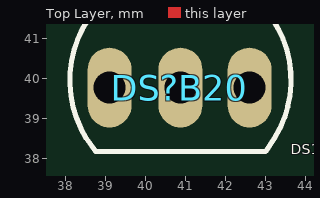
[diagram p0: Top Layer view]
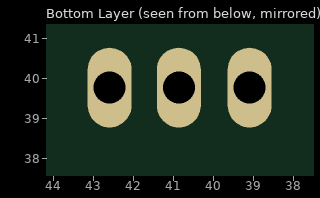
[diagram p1: Bottom Layer view, seen from below]
# Altium PCB MISC84237-4.PcbDoc
Units mm, origin at the board's own origin, x right, y up, seen from the top; angles counter-clockwise.
Board outline 32.45 x 30.27 mm, 2 copper layers (Top Layer, Bottom Layer); 1 components, 0 nets, 3 pads, 0 vias.

## Layer stack, top to bottom (the 12.6 mil dielectric is the usual default, probably not edited)
Top Layer: signal copper (thickness not stored)
Dielectric: dielectric 0.32, FR-4, Dk 4.8
Bottom Layer: signal copper (thickness not stored)

## Board outline
57.852,25.4 25.4,25.4 25.4,55.668 57.852,55.668

## Components (designator, comment, footprint, x,y, rotation, side; value= is the part's Value field where it differs from the comment)
DS?B20 "DS18B20 temperature sensor" DS18B20温度传感器 40.864,40.407 r0 top

## Footprints (in the part's own frame and the unit in brackets; to place one, negate y for a bottom-side part, rotate by r counter-clockwise, add the part's x,y. Pads: shape width x height; smd on the part's side, far side on the other; paste and mask are expansions set on the pad)
DS18B20温度传感器 [mm]
  oval 1.1x2 hole 0.8 paste+0 mask+0.051: 1(-1.77,-0.643) 2(0,-0.643) 3(1.73,-0.643)
  silkscreen extent -2.76,-2.24 2.76,2.3

## Nets (pads, with @x,y where several pads share a name; then routed paths per layer and width w, separated by ;. In a path a pad name is that pad's centre, name@x,y a point inside that pad or via, vN(x,y) a via of type N, cw(c..) or ccw(c..) an arc to the next point about the centre after c; other vN are vias at no path point)
pads on no net: DS?B20.1 DS?B20.2 DS?B20.3

## Silkscreen, mask and mechanical layers (free items; w line width, h text height)
Document:
  lines w0.003: 41.626,40.534 41.626,40.534